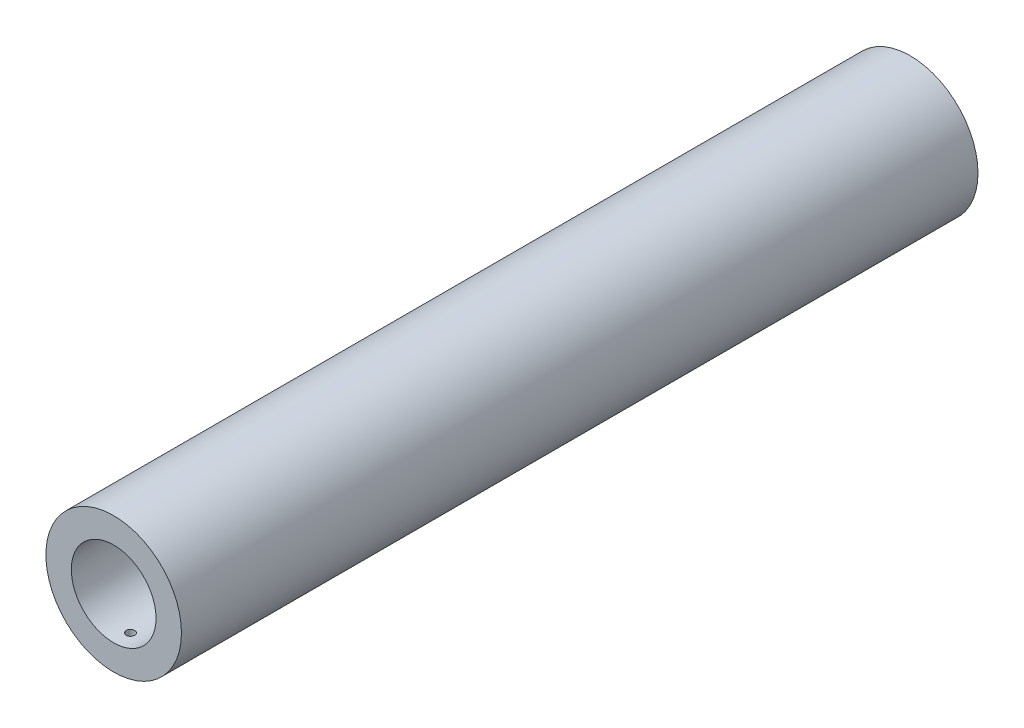
SolidWorks part; units mm, degrees
ref_plane "Front Plane" through (0, 0, 0) normal (0, 0, 1) x (1, 0, 0)
ref_plane "Top Plane" through (0, 0, 0) normal (0, 1, 0) x (1, 0, 0)
ref_plane "Right Plane" through (0, 0, 0) normal (1, 0, 0) x (0, 0, -1)
other "Configuration Table"
sketch "Sketch1" plane through (0, 0, 0) normal (0, 0, 1) x (1, 0, 0)
  circle A0 centre (0, 0) radius 40
  circle A1 centre (0, 0) radius 25
  dimension "D1" = 80
  dimension "D2" = 50
extrude "Boss-Extrude1" add sketch "Sketch1" along normal blind 470
sketch "Sketch2" plane through (0, 0, 0) normal (0, 1, 0) x (1, 0, 0)
  line L0 (40, 0) -> (-40, 0) construction
  line L1 (-40, -470) -> (40, -470) construction
  circle A0 centre (0, -460) radius 2.5
  circle A1 centre (0, -10) radius 2.5
  dimension "D1" = 5
  dimension "D2" = 10
  dimension "D3" = 5
  dimension "D4" = 10
extrude "Cut-Extrude1" cut sketch "Sketch2" against normal up to next
